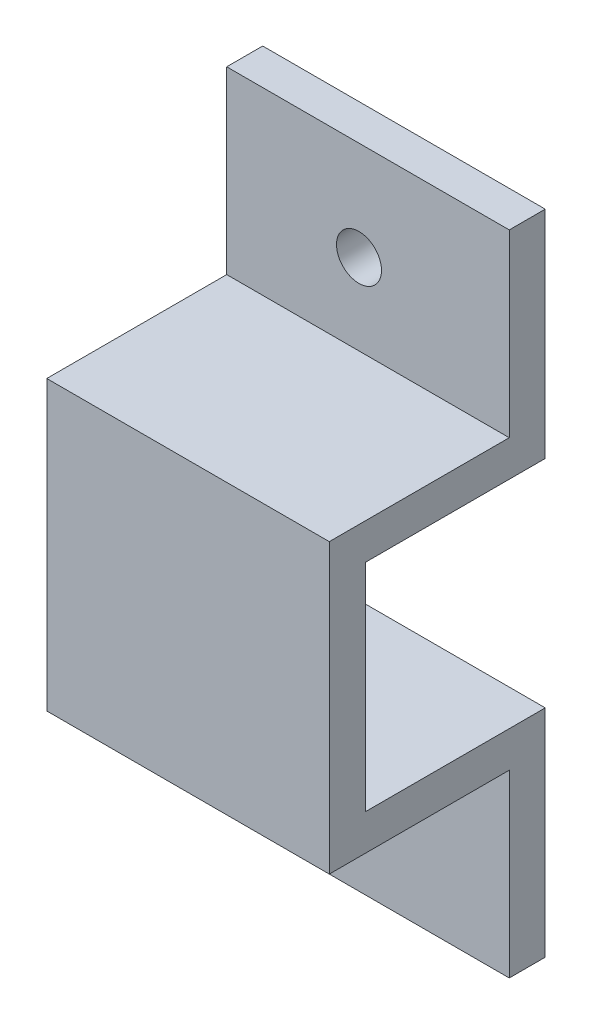
from build123d import *

# Parameters (mm, degrees)
SKETCH1_W           = 16.7
SKETCH1_H           = 12
BOSS_EXTRUDE1_DEPTH = 2
SKETCH2_W           = 16.7
SKETCH2_H           = 2
BOSS_EXTRUDE2_DEPTH = 12
SKETCH4_W           = 2
SKETCH4_H           = 10
BOSS_EXTRUDE3_DEPTH = 16.7
M3_TAPPED_HOLE1_D   = 2.5
CUT_EXTRUDE1_DEPTH  = 1


with BuildPart() as part:
    # Sketch1 → Boss-Extrude1 (new body)
    with BuildSketch(Plane.XY):
        Rectangle(SKETCH1_W, SKETCH1_H)
    extrude(amount=BOSS_EXTRUDE1_DEPTH)

    # Sketch2 → Boss-Extrude2 (add)
    with BuildSketch(Plane.XY.offset(2)):
        with Locations((0, 7)):
            Rectangle(SKETCH2_W, SKETCH2_H)
        with Locations((0, -7)):
            Rectangle(SKETCH2_W, SKETCH2_H)
    extrude(amount=-BOSS_EXTRUDE2_DEPTH)

    # Sketch4 → Boss-Extrude3 (add)
    with BuildSketch(Plane.ZY.offset(8.35)):
        with Locations((-9, -13)):
            Rectangle(SKETCH4_W, SKETCH4_H)
        with Locations((-9, 13)):
            Rectangle(SKETCH4_W, SKETCH4_H)
    extrude(amount=-BOSS_EXTRUDE3_DEPTH)

    # M3 Tapped Hole1 (through all)
    with Locations(Plane.XY.offset(-8)):
        with Locations((0, -12.5), (0, 12.5)):
            Hole(M3_TAPPED_HOLE1_D / 2)

    # Sketch8 → Cut-Extrude1 (cut)
    with BuildSketch(Plane.ZY.offset(8.35)):
        Polygon((0, 6), (0, -6), (-10, -6), (-10, -18), (-8, -18), (-8, -8), (2, -8), (2, 8), (-8, 8), (-8, 18), (-10, 18), (-10, 6), align=None)
    extrude(amount=-CUT_EXTRUDE1_DEPTH, mode=Mode.SUBTRACT)


solid = part.part
